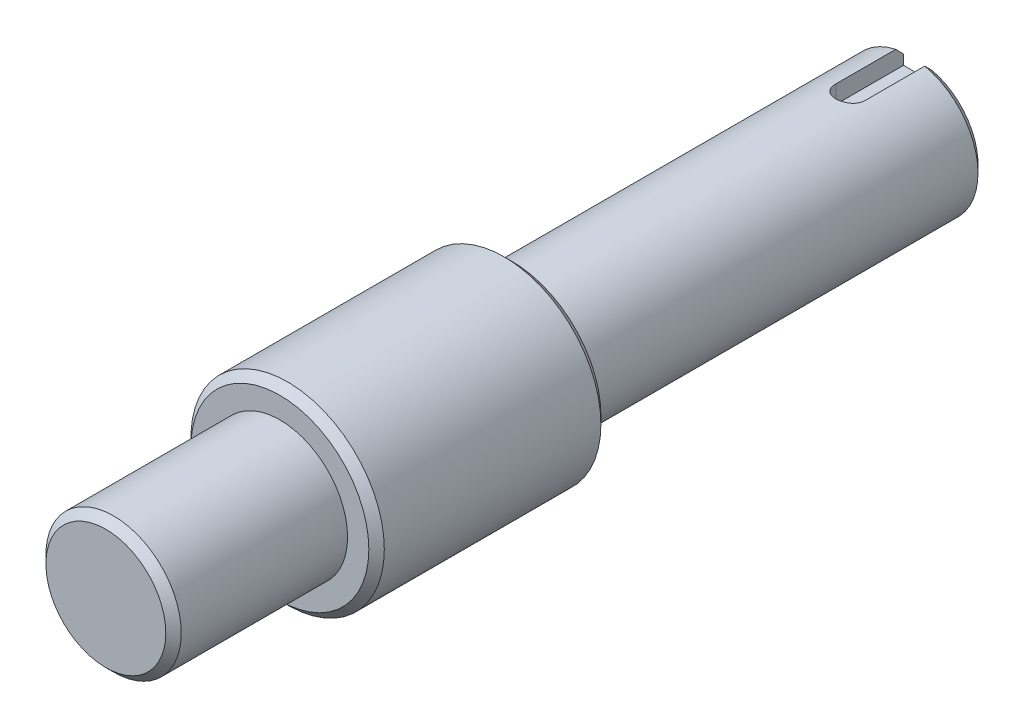
SolidWorks part; units mm, degrees
ref_plane "Front Plane" through (0, 0, 0) normal (0, 0, 1) x (1, 0, 0)
ref_plane "Top Plane" through (0, 0, 0) normal (0, 1, 0) x (1, 0, 0)
ref_plane "Right Plane" through (0, 0, 0) normal (1, 0, 0) x (0, 0, -1)
sketch "Sketch1" plane through (0, 0, 0) normal (0, 0, 1) x (1, 0, 0)
  circle A0 centre (0, 0) radius 35
  dimension "D1" = 70
extrude "Boss-Extrude1" add sketch "Sketch1" along normal blind 150 and the other way blind 270
sketch "Sketch2" plane through (0, 0, 0) normal (0, 0, 1) x (1, 0, 0)
  circle A0 centre (0, 0) radius 50
  dimension "D1" = 100
extrude "Boss-Extrude2" add sketch "Sketch2" along normal mid plane 120
ref_plane "Plane1" through (0, 35, 0) normal (0, 1, 0) x (1, 0, 0)
chamfer "Chamfer1" distance 4 angle 45 4 edges at (35, 0, -270) (50, 0, 60) (50, 0, -60) (35, 0, 150)
sketch "Sketch3" plane through (0, 35, 0) normal (0, 1, 0) x (1, 0, 0)
  line L0 (0, 282.6601) -> (0, 0) construction
  line L1 (35, 270) -> (-35, 270) construction
  line L2 (-7.5, 305) -> (7.5, 305)
  line L3 (-7.5, 305) -> (-7.5, 235)
  line L5 (7.5, 305) -> (7.5, 235)
  line L6 (-7.5, 305) -> (7.5, 235) construction
  line L7 (-7.5, 235) -> (7.5, 305) construction
  arc A0 (-7.5, 235) -> (7.5, 235) centre (0, 235) ccw
  point P3 (0, 270)
  dimension "D1" = 15
  dimension "D2" = 70
extrude "Cut-Extrude1" cut sketch "Sketch3" against normal blind 10
